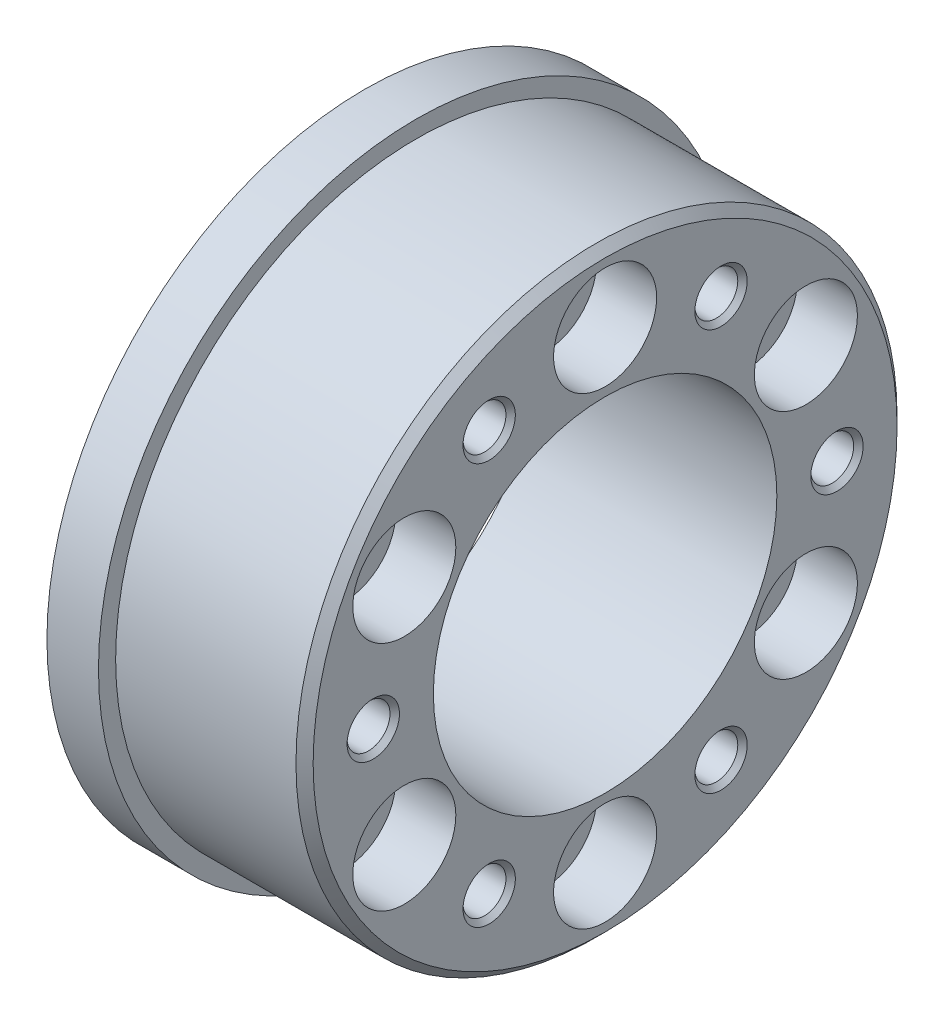
SolidWorks part; units mm, degrees
material "6061 合金"
ref_plane "前视基准面" through (0, 0, 0) normal (0, 0, 1) x (1, 0, 0)
ref_plane "上视基准面" through (0, 0, 0) normal (0, 1, 0) x (1, 0, 0)
ref_plane "右视基准面" through (0, 0, 0) normal (1, 0, 0) x (0, 0, -1)
other "Configuration Table"
sketch "草图1" plane through (0, 0, 0) normal (0, 1, 0) x (1, 0, 0)
  line L0 (-415.5917, 0) -> (20363.994, 0) construction
  line L2 (0, 18.5) -> (3, 18.5)
  line L3 (3, 18.5) -> (3, 17.5)
  line L4 (3, 17.5) -> (14, 17.5)
  line L5 (14, 17.5) -> (14, 10)
  line L7 (14, 10) -> (0, 10)
  line L10 (0, 18.5) -> (0, 10)
  dimension "D1" = 20
  dimension "D2" = 35
  dimension "D3" = 37
  dimension "D4" = 11
  dimension "D5" = 3
revolve "旋转1" add sketch "草图1" angle 360 about L0
sketch "草图2" plane through (14, 0, 0) normal (1, 0, 0) x (0, 0, -1)
  circle A0 centre (0, 0) radius 13.5 construction
  circle A1 centre (0, 13.5) radius 1.6
  circle A2 centre (11.6913, 6.75) radius 1.6
  circle A3 centre (11.6913, -6.75) radius 1.6
  circle A4 centre (0, -13.5) radius 1.6
  circle A5 centre (-11.6913, -6.75) radius 1.6
  circle A6 centre (-11.6913, 6.75) radius 1.6
  point P18 (0, 0)
  dimension "D1" = 27
  dimension "D2" = 3.2
  dimension "D3" = 6
extrude "切除-拉伸1" cut sketch "草图2" against normal through all
chamfer "倒角1" distance 0.5 angle 45 1 edges at (14, 0, 17.5)
sketch "草图3" plane through (14, 0, 0) normal (1, 0, 0) x (0, 0, -1)
  circle A0 centre (0, 13.5) radius 3
  circle A1 centre (11.6913, 6.75) radius 3
  circle A2 centre (11.6913, -6.75) radius 3
  circle A3 centre (0, -13.5) radius 3
  circle A4 centre (-11.6913, -6.75) radius 3
  circle A5 centre (-11.6913, 6.75) radius 3
  point P16 (0, 0)
  dimension "D1" = 6
  dimension "D2" = 6
extrude "切除-拉伸2" cut sketch "草图3" against normal blind 3.5
sketch "草图4" plane through (14, 0, 0) normal (1, 0, 0) x (0, 0, -1)
  line L0 (0, 13.5) -> (0, 0) construction
  line L1 (0, 0) -> (6.75, 11.6913) construction
  circle A0 centre (0, 0) radius 13.5 construction
  point P3 (6.75, 11.6913)
  point P7 (13.5, 0)
  point P10 (6.75, -11.6913)
  point P11 (-6.75, -11.6913)
  point P12 (-13.5, 0)
  point P13 (-6.75, 11.6913)
  dimension "D1" = 27
  dimension "D2" = 30
  dimension "D3" = 6
hole_wizard "M3 螺纹孔1" positions "草图4" profile "草图5" tap size "M3" standard "GB" end condition through all
sketch "草图5" plane through (14, 11.6913, 6.75) normal (0, 1, 0) x (0, 0, -1)
  line L0 (0, 0) -> (0, 14)
  line L1 (0, 14) -> (1.25, 14)
  line L2 (1.25, 14) -> (1.25, 0.275)
  line L3 (1.25, 0.275) -> (1.525, 0)
  line L5 (1.525, 0) -> (0, 0)
  line L6 (-1.25, 0.275) -> (-1.525, 0) construction
  line L11 (0, -6.35) -> (0, 107.95) construction
  dimension "通孔螺纹孔钻头直径" = 2.5
  dimension "通孔螺纹孔钻头深度" = 14
  dimension "近端锥形沉头孔直径" = 3.05
  dimension "近端锥形沉头孔角度" = 90
cosmetic thread "孔螺纹线1" parameters "D2"=3
cosmetic thread "孔螺纹线2" parameters "D2"=3
cosmetic thread "孔螺纹线3" parameters "D2"=3
cosmetic thread "孔螺纹线4" parameters "D2"=3
cosmetic thread "孔螺纹线5" parameters "D2"=3
cosmetic thread "孔螺纹线6" parameters "D2"=3
